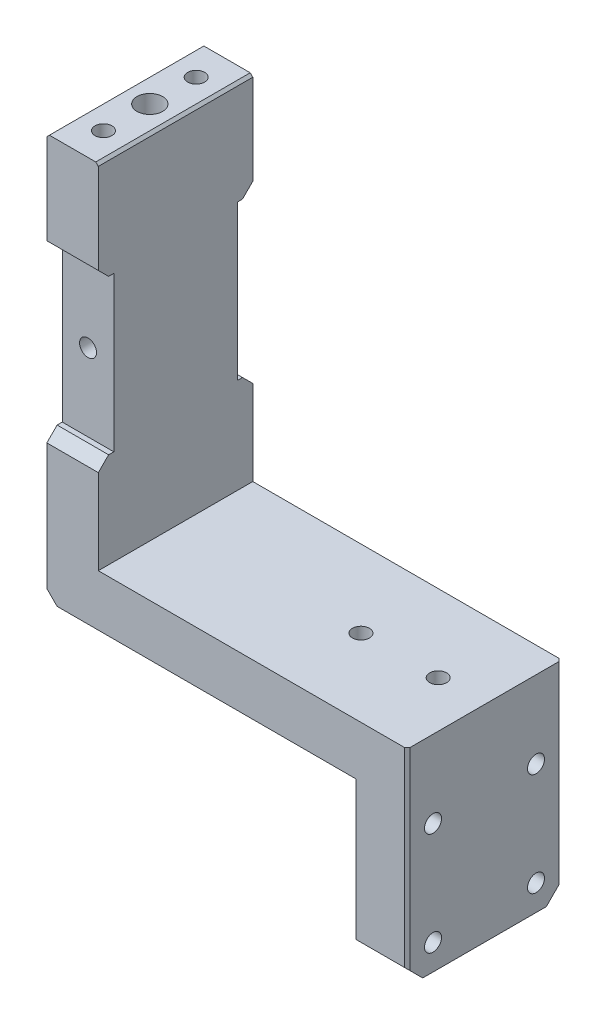
from build123d import *

# Parameters (mm, degrees)
SKETCH1_W             = 70
SKETCH1_H             = 40
BOSS_EXTRUDE1_DEPTH   = 15
SKETCH2_W             = 60
SKETCH2_H             = 30
CUT_EXTRUDE1_DEPTH    = 51.249378106
CHAMFER1_SIZE         = 0.5
M4_TAPPED_HOLE1_D     = 3.3
M4_TAPPED_HOLE1_DEPTH = 11.5
M4_TAPPED_HOLE1_TIP   = 0.991420021
M4_TAPPED_HOLE2_D     = 3.3
CHAMFER3_SIZE         = 3
SKETCH17_W            = 10
SKETCH17_H            = 30
BOSS_EXTRUDE2_DEPTH   = 68.5
CHAMFER4_SIZE         = 0.5
M4_TAPPED_HOLE3_D     = 3.3
M4_TAPPED_HOLE3_DEPTH = 11.5
M4_TAPPED_HOLE3_TIP   = 0.991420021
CHAMFER5_SIZE         = 2
SKETCH20_R            = 2.5
CUT_EXTRUDE2_DEPTH    = 8
SKETCH21_W            = 3
SKETCH21_H            = 30
CUT_EXTRUDE3_DEPTH    = 114.829916981
CHAMFER6_SIZE         = 2


with BuildPart() as part:
    # Sketch1 → Boss-Extrude1 (new, symmetric)
    with BuildSketch(Plane.XY):
        Rectangle(SKETCH1_W, SKETCH1_H)
    extrude(amount=BOSS_EXTRUDE1_DEPTH, both=True)

    # Sketch2 → Cut-Extrude1 (cut, through all)
    with BuildSketch(Plane.XY.offset(15)):
        with Locations((-5, -5)):
            Rectangle(SKETCH2_W, SKETCH2_H)
    extrude(amount=-CUT_EXTRUDE1_DEPTH, mode=Mode.SUBTRACT)

    # Chamfer1
    chamfer1_edges = [part.edges().sort_by_distance(p)[0] for p in [
        (35, 0, 15),
        (35, 0, -15),
    ]]
    chamfer(chamfer1_edges, length=CHAMFER1_SIZE)

    # M4 Tapped Hole1
    with Locations(Plane(origin=(0, 20, 0), x_dir=(1, 0, 0), z_dir=(0, 1, 0))):
        with Locations((11, 0), (26, 0)):
            Hole(M4_TAPPED_HOLE1_D / 2, depth=M4_TAPPED_HOLE1_DEPTH)
            with Locations((0, 0, -(M4_TAPPED_HOLE1_DEPTH + M4_TAPPED_HOLE1_TIP / 2))):  # 118° drill point
                Cone(0, M4_TAPPED_HOLE1_D / 2, M4_TAPPED_HOLE1_TIP, mode=Mode.SUBTRACT)

    # M4 Tapped Hole2 (through all)
    with Locations(Plane(origin=(35, 0, 0), x_dir=(0, 0, -1), z_dir=(1, 0, 0))):
        with Locations((-10, 5), (-10, -15), (10, -15), (10, 5)):
            Hole(M4_TAPPED_HOLE2_D / 2)

    # Chamfer3
    chamfer3_edges = [part.edges().sort_by_distance(p)[0] for p in [
        (29.75, -20, -15),
        (29.75, -20, 15),
    ]]
    chamfer(chamfer3_edges, length=CHAMFER3_SIZE)

    # Sketch17 → Boss-Extrude2 (add)
    with BuildSketch(Plane(origin=(0, 20, 0), x_dir=(1, 0, 0), z_dir=(0, 1, 0))):
        with Locations((-30, 0)):
            Rectangle(SKETCH17_W, SKETCH17_H)
    extrude(amount=BOSS_EXTRUDE2_DEPTH)

    # Chamfer4
    chamfer4_edges = [part.edges().sort_by_distance(p)[0] for p in [
        (-25, 88.5, 0),
        (-35, 88.5, 0),
    ]]
    chamfer(chamfer4_edges, length=CHAMFER4_SIZE)

    # M4 Tapped Hole3
    with Locations(Plane(origin=(0, 88.5, 0), x_dir=(1, 0, 0), z_dir=(0, 1, 0))):
        with Locations((-30, 9), (-30, -9)):
            Hole(M4_TAPPED_HOLE3_D / 2, depth=M4_TAPPED_HOLE3_DEPTH)
            with Locations((0, 0, -(M4_TAPPED_HOLE3_DEPTH + M4_TAPPED_HOLE3_TIP / 2))):  # 118° drill point
                Cone(0, M4_TAPPED_HOLE3_D / 2, M4_TAPPED_HOLE3_TIP, mode=Mode.SUBTRACT)

    # Chamfer5
    chamfer5_edges = [part.edges().sort_by_distance(p)[0] for p in [
        (-35, 10, 0),
    ]]
    chamfer(chamfer5_edges, length=CHAMFER5_SIZE)

    # Sketch20 → Cut-Extrude2 (cut)
    with BuildSketch(Plane(origin=(0, 88.5, 0), x_dir=(1, 0, 0), z_dir=(0, 1, 0))):
        with Locations(Location((-30, 0, 0), (0, 0, 270))):
            Circle(SKETCH20_R)
    extrude(amount=-CUT_EXTRUDE2_DEPTH, mode=Mode.SUBTRACT)

    # Sketch21 → Cut-Extrude3 (cut, through all)
    with BuildSketch(Plane.ZY.offset(35)):
        with Locations((-13.5, 53.5)):
            Rectangle(SKETCH21_W, SKETCH21_H)
    cut_extrude3 = extrude(amount=-CUT_EXTRUDE3_DEPTH, mode=Mode.SUBTRACT)

    # Sketch22 → M4 Tapped Hole4 (revolve, cut)
    with BuildSketch(Plane(origin=(-30, 53.5, -12), x_dir=(0, 1, 0), z_dir=(1, 0, 0))):
        Polygon((0, 0), (0, 12.491420021), (1.65, 11.5), (1.65, 0), align=None)
    m4_tapped_hole4 = revolve(axis=Axis((-30, 53.5, -18.35), (0, 0, 1)), mode=Mode.SUBTRACT)

    # Mirror2: Cut-Extrude3, M4 Tapped Hole4 across plane
    add(cut_extrude3.mirror(Plane.XY), mode=Mode.SUBTRACT)
    add(m4_tapped_hole4.mirror(Plane.XY), mode=Mode.SUBTRACT)

    # Chamfer6
    chamfer6_edges = [part.edges().sort_by_distance(p)[0] for p in [
        (-30, 38.5, -15),
        (-30, 68.5, -15),
        (-30, 68.5, 15),
        (-30, 38.5, 15),
    ]]
    chamfer(chamfer6_edges, length=CHAMFER6_SIZE)


solid = part.part
